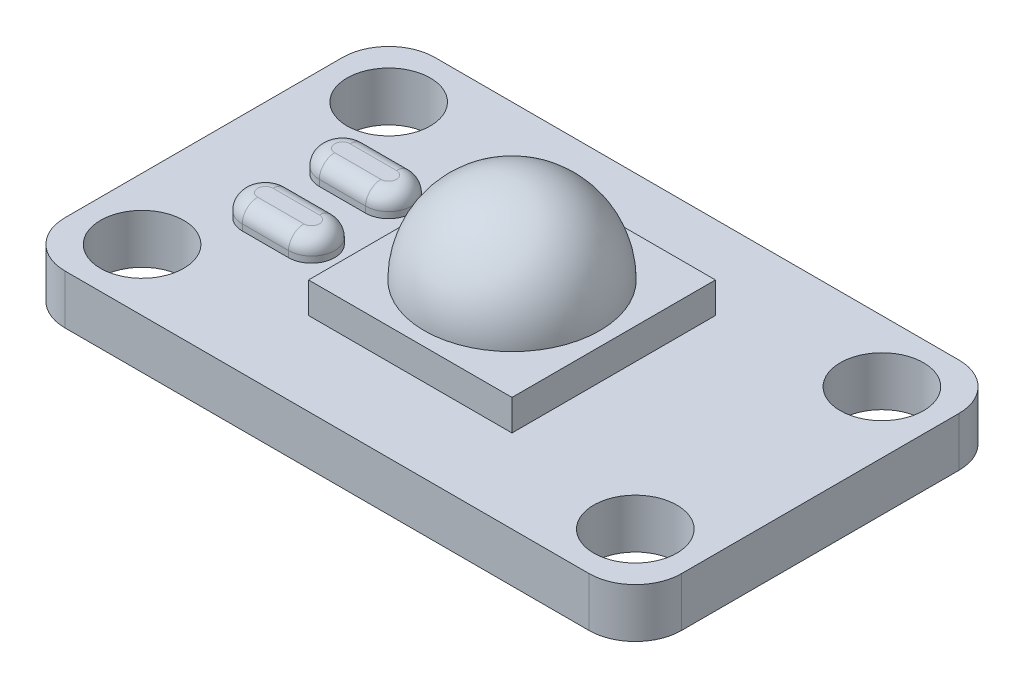
from build123d import *

# Parameters (mm, degrees)
ALUMINIUM_BASE_PLATE_DEPTH        = 1.6
SKETCH7_R                         = 1.35
SCREW_HOLE_DEPTH                  = 12.771151176
SKETCH_587_W                      = 6.6
SKETCH_587_H                      = 6.6
LED_BEAD_BOARD_DEPTH              = 1
SOLDER_JOINT_BASE_OUTLINE_DEPTH   = 0.7
SOLDER_JOINT_BASE_OUTLINE_2_DEPTH = 0.7
SOLDER_JOINT_1_R                  = 0.5
SOLDER_JOINT_2_R                  = 0.5


with BuildPart() as part:
    # Aluminium base plate outline → Aluminium base plate (new body)
    with BuildSketch(Plane(origin=(0, 0, 0), x_dir=(1, 0, 0), z_dir=(0, 1, 0))):
        with BuildLine():
            Line((-8.5, -6), (8.5, -6))
            ThreePointArc((8.5, -6), (9.560660172, -5.560660172), (10, -4.5))
            Line((10, -4.5), (10, 4.5))
            ThreePointArc((10, 4.5), (9.560660172, 5.560660172), (8.5, 6))
            Line((8.5, 6), (-8.5, 6))
            ThreePointArc((-8.5, 6), (-9.560660172, 5.560660172), (-10, 4.5))
            Line((-10, 4.5), (-10, -4.5))
            ThreePointArc((-10, -4.5), (-9.560660172, -5.560660172), (-8.5, -6))
        make_face()
    extrude(amount=ALUMINIUM_BASE_PLATE_DEPTH)

    # Sketch7 → Screw hole (cut, through all)
    with BuildSketch(Plane(origin=(0, 0, 0), x_dir=(1, 0, 0), z_dir=(0, 1, 0))):
        with Locations(Location((-8, -4, 0), (0, 0, 270))):
            Circle(SKETCH7_R)
        with Locations(Location((8, -4, 0), (0, 0, 270))):
            Circle(SKETCH7_R)
        with Locations(Location((8, 4, 0), (0, 0, 270))):
            Circle(SKETCH7_R)
        with Locations(Location((-8, 4, 0), (0, 0, 270))):
            Circle(SKETCH7_R)
    extrude(amount=SCREW_HOLE_DEPTH, mode=Mode.SUBTRACT)


with BuildPart() as body_2:
    # Sketch 587 → LED bead board (new body)
    with BuildSketch(Plane(origin=(0, 1.6, 0), x_dir=(1, 0, 0), z_dir=(0, 1, 0))):
        Rectangle(SKETCH_587_W, SKETCH_587_H)
    extrude(amount=LED_BEAD_BOARD_DEPTH)

    # LED bead rotation base → LED bead (revolve)
    with BuildSketch(Plane.XY):
        with BuildLine():
            Line((0, 2.6), (2.85, 2.6))
            ThreePointArc((2.85, 2.6), (2.015254326, 4.615254326), (0, 5.45))
            Line((0, 5.45), (0, 2.6))
        make_face()
    revolve(axis=Axis((0, 2.6, 0), (0, 1, 0)))


with BuildPart() as body_3:
    # Solder pad → Solder joint base outline (new body)
    with BuildSketch(Plane(origin=(0, 1.6, 0), x_dir=(1, 0, 0), z_dir=(0, 1, 0))):
        with BuildLine():
            Line((-6.75, 2), (-5.25, 2))
            ThreePointArc((-5.25, 2), (-4.5, 1.25), (-5.25, 0.5))
            Line((-5.25, 0.5), (-6.75, 0.5))
            ThreePointArc((-6.75, 0.5), (-7.5, 1.25), (-6.75, 2))
        make_face()
    extrude(amount=SOLDER_JOINT_BASE_OUTLINE_DEPTH)

    # Solder joint 1
    solder_joint_1_edges = [body_3.edges().sort_by_distance(p)[0] for p in [
        (-4.5, 2.3, -1.25),
        (-6, 2.3, -2),
        (-7.5, 2.3, -1.25),
        (-6, 2.3, -0.5),
    ]]
    fillet(solder_joint_1_edges, radius=SOLDER_JOINT_1_R)


with BuildPart() as body_4:
    # Solder pad → Solder joint base outline 2 (new body)
    with BuildSketch(Plane(origin=(0, 1.6, 0), x_dir=(1, 0, 0), z_dir=(0, 1, 0))):
        with BuildLine():
            Line((-6.75, -0.5), (-5.25, -0.5))
            ThreePointArc((-5.25, -0.5), (-4.5, -1.25), (-5.25, -2))
            Line((-5.25, -2), (-6.75, -2))
            ThreePointArc((-6.75, -2), (-7.5, -1.25), (-6.75, -0.5))
        make_face()
    extrude(amount=SOLDER_JOINT_BASE_OUTLINE_2_DEPTH)

    # Solder joint 2
    solder_joint_2_edges = [body_4.edges().sort_by_distance(p)[0] for p in [
        (-7.5, 2.3, 1.25),
        (-6, 2.3, 2),
        (-4.5, 2.3, 1.25),
        (-6, 2.3, 0.5),
    ]]
    fillet(solder_joint_2_edges, radius=SOLDER_JOINT_2_R)


solid = Compound([part.part, body_2.part, body_3.part, body_4.part])
